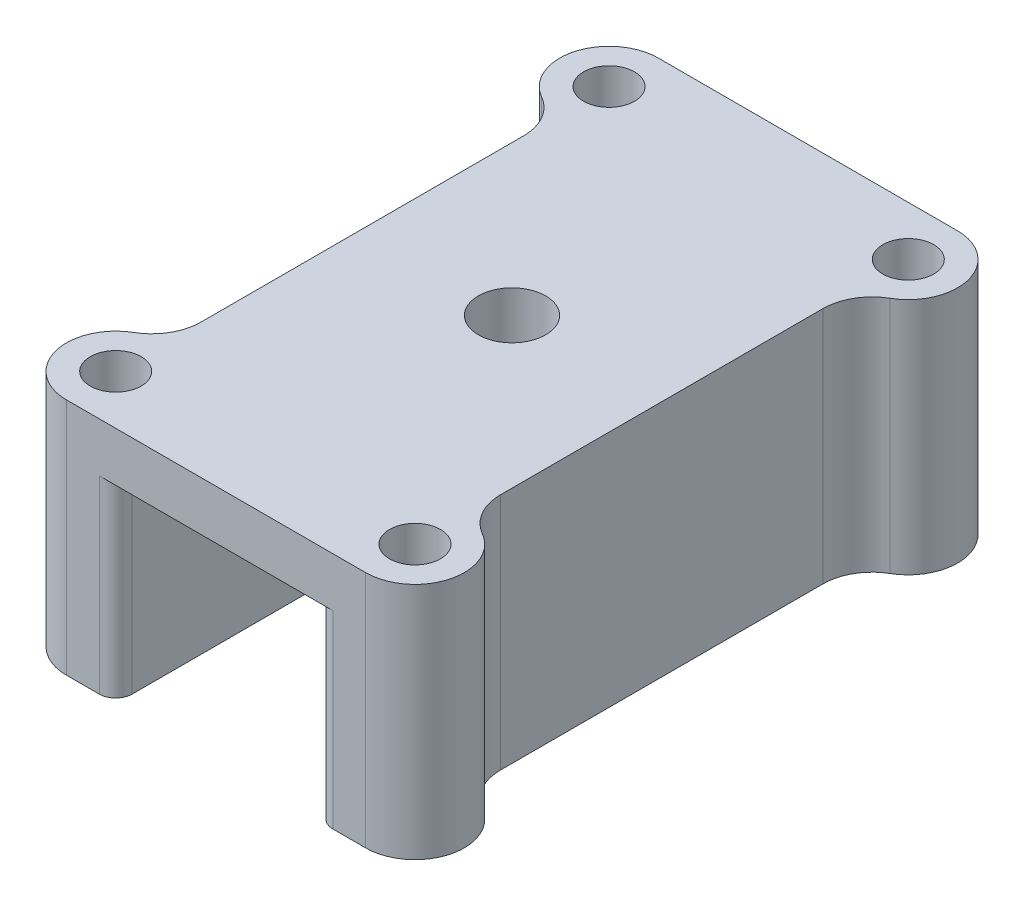
SolidWorks part; units mm, degrees
material "6061 合金"
ref_plane "前视基准面" through (0, 0, 0) normal (0, 0, 1) x (1, 0, 0)
ref_plane "上视基准面" through (0, 0, 0) normal (0, 1, 0) x (1, 0, 0)
ref_plane "右视基准面" through (0, 0, 0) normal (1, 0, 0) x (0, 0, -1)
sketch "草图1" plane through (0, 0, 0) normal (0, 0, 1) x (1, 0, 0)
  line L0 (-6.1, 6) -> (6.1, 6)
  line L1 (-6, 6) -> (6, 6) construction
  line L2 (-6, 6) -> (-6, -6) construction
  line L3 (-6, -6) -> (6, -6) construction
  line L4 (6, 6) -> (6, -6) construction
  line L5 (-6, 6) -> (6, -6) construction
  line L6 (-6, -6) -> (6, 6) construction
  line L7 (-6.1, 6) -> (-6.1, -5.5)
  line L8 (-6.1, -5.5) -> (-9.1, -5.5)
  line L9 (-9.1, -5.5) -> (-9.1, 9)
  line L10 (-9.1, 9) -> (9.1, 9)
  line L11 (9.1, 9) -> (9.1, -5.5)
  line L12 (9.1, -5.5) -> (6.1, -5.5)
  line L13 (6.1, -5.5) -> (6.1, 6)
  point P0 (0, 0)
  dimension "D1" = 12
  dimension "D2" = 0.1
  dimension "D3" = 0.1
  dimension "D4" = 3
  dimension "D5" = 3
  dimension "D6" = 0.5
extrude "凸台-拉伸1" add sketch "草图1" along normal blind 36
sketch "草图2" plane through (0, 9, 0) normal (0, 1, 0) x (1, 0, 0)
  line L0 (6, 3.5949) -> (6, -40.4406) construction
  line L1 (-26.5482, -18) -> (27.5147, -18) construction
  line L2 (9.1, 0) -> (-9.1, 0) construction
  line L3 (9.1, -36) -> (9.1, 0) construction
  line L4 (-9.1, -36) -> (-9.1, 0) construction
  circle A0 centre (9.1, -3) radius 3
  circle A2 centre (-9.1, -3) radius 3
  circle A3 centre (9.1, -33) radius 3
  circle A4 centre (-9.1, -33) radius 3
  dimension "D3" = 6
  dimension "D4" = 15
  dimension "D1" = 6
  dimension "D2" = 18
extrude "凸台-拉伸2" add sketch "草图2" against normal up to surface (14.5 mm away) up to face at (-7.6, -5.5, 18)
sketch "草图3" plane through (0, 9, 0) normal (0, 1, 0) x (1, 0, 0)
  line L0 (9.1, 0) -> (-9.1, 0) construction
  circle A0 centre (9.1, -3) radius 1.55
  arc A1 (9.1, -6) -> (9.1, 0) centre (9.1, -3) ccw construction
  circle A2 centre (-9.1, -33) radius 1.55
  circle A3 centre (9.1, -33) radius 1.55
  circle A4 centre (-9.1, -3) radius 1.55
  arc A5 (-9.1, 0) -> (-9.1, -6) centre (-9.1, -3) ccw construction
  arc A6 (-9.1, -30) -> (-9.1, -36) centre (-9.1, -33) ccw construction
  arc A7 (9.1, -36) -> (9.1, -30) centre (9.1, -33) ccw construction
  circle A8 centre (0, -18) radius 2.05
  dimension "D1" = 3.1
  dimension "D2" = 4.1
  dimension "D3" = 18
extrude "切除-拉伸1" cut sketch "草图3" against normal through all
fillet "圆角1" radius 3 4 edges at (-9.1, 1.75, 6) (-9.1, 1.75, 30) (9.1, 1.75, 6) (9.1, 1.75, 30)
fillet "圆角2" radius 1 4 edges at (6.1, 0.25, 0) (-6.1, 0.25, 0) (6.1, 0.25, 36) (-6.1, 0.25, 36)
